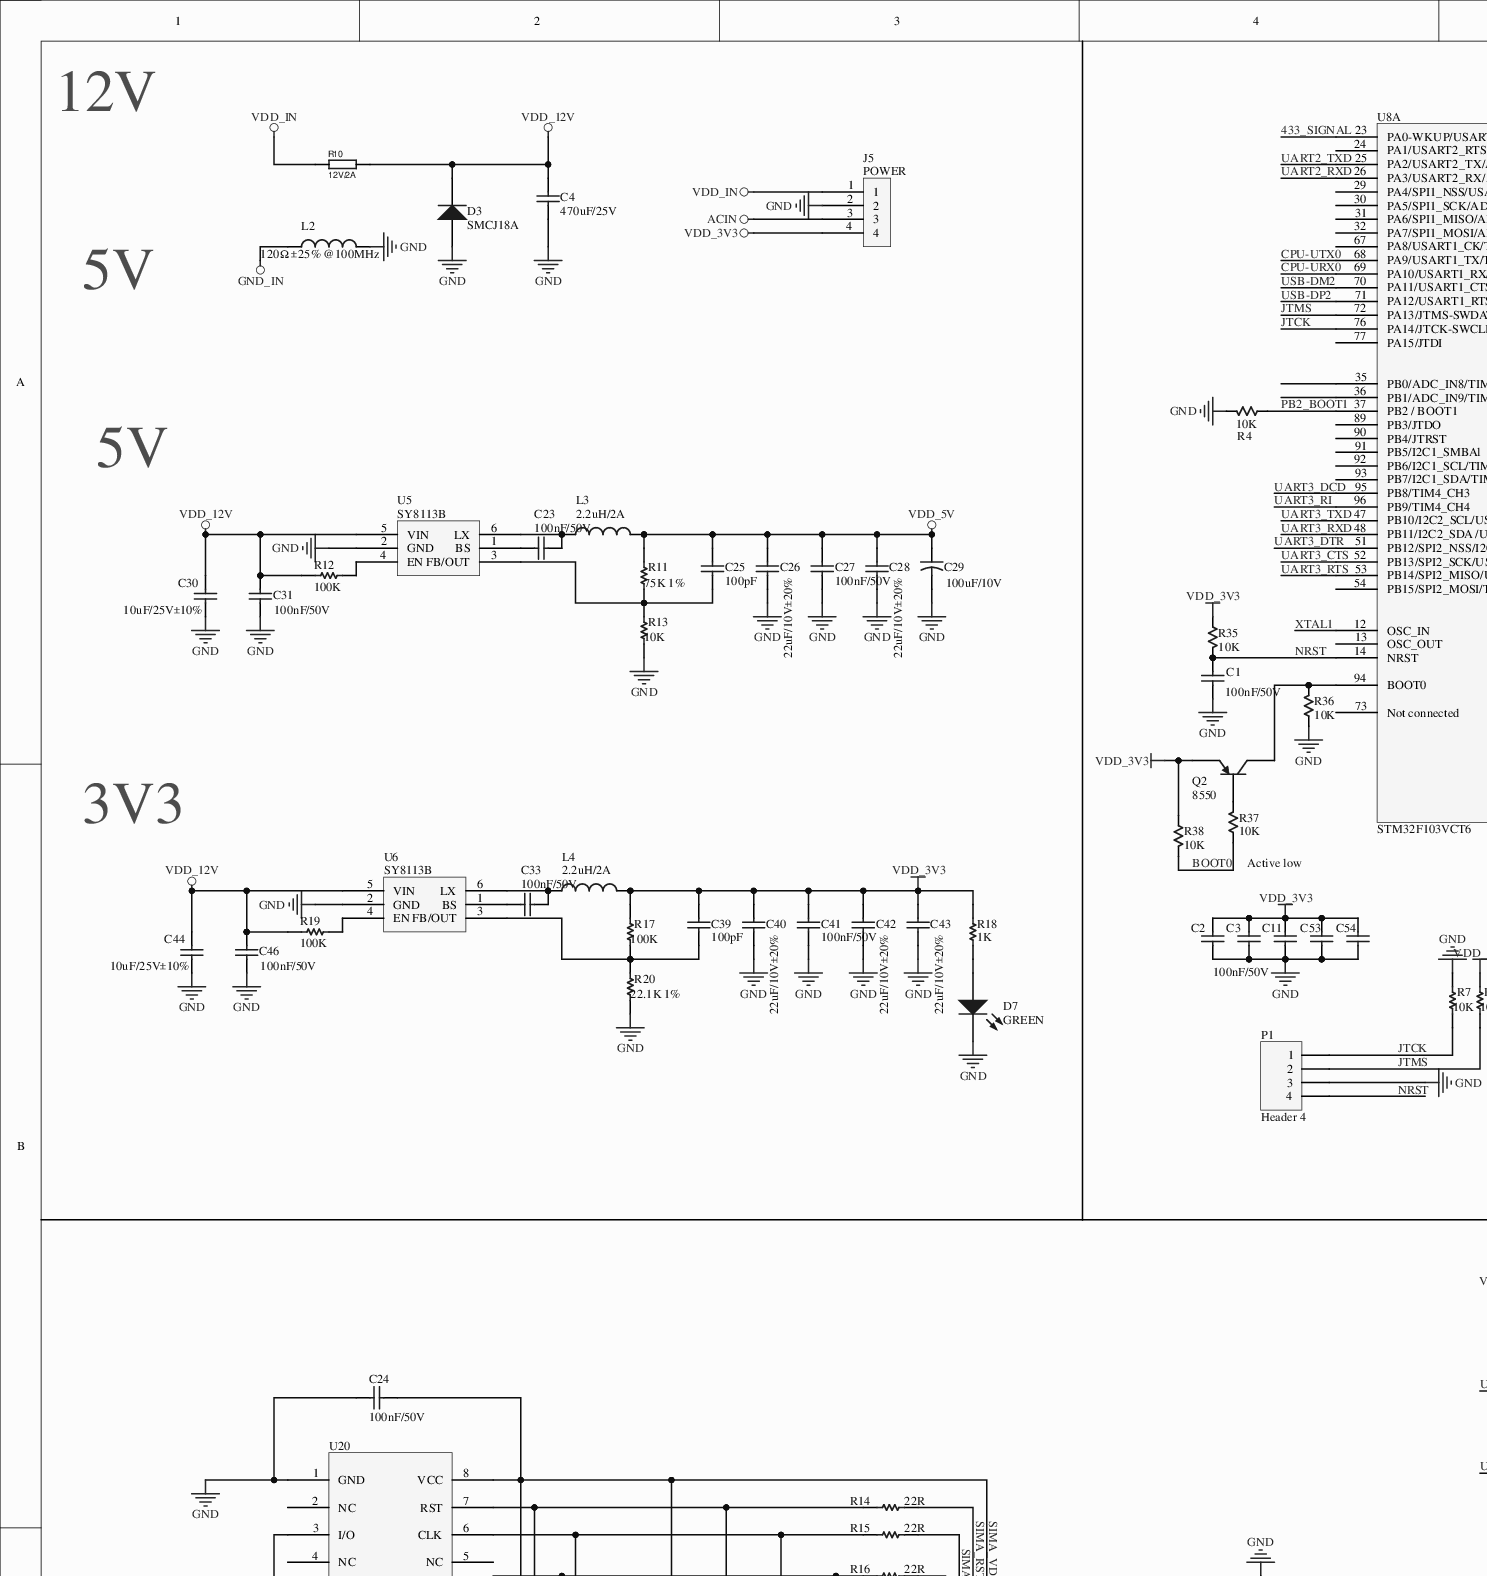
[diagram p0: MISC84456-4.SchDoc, top left]
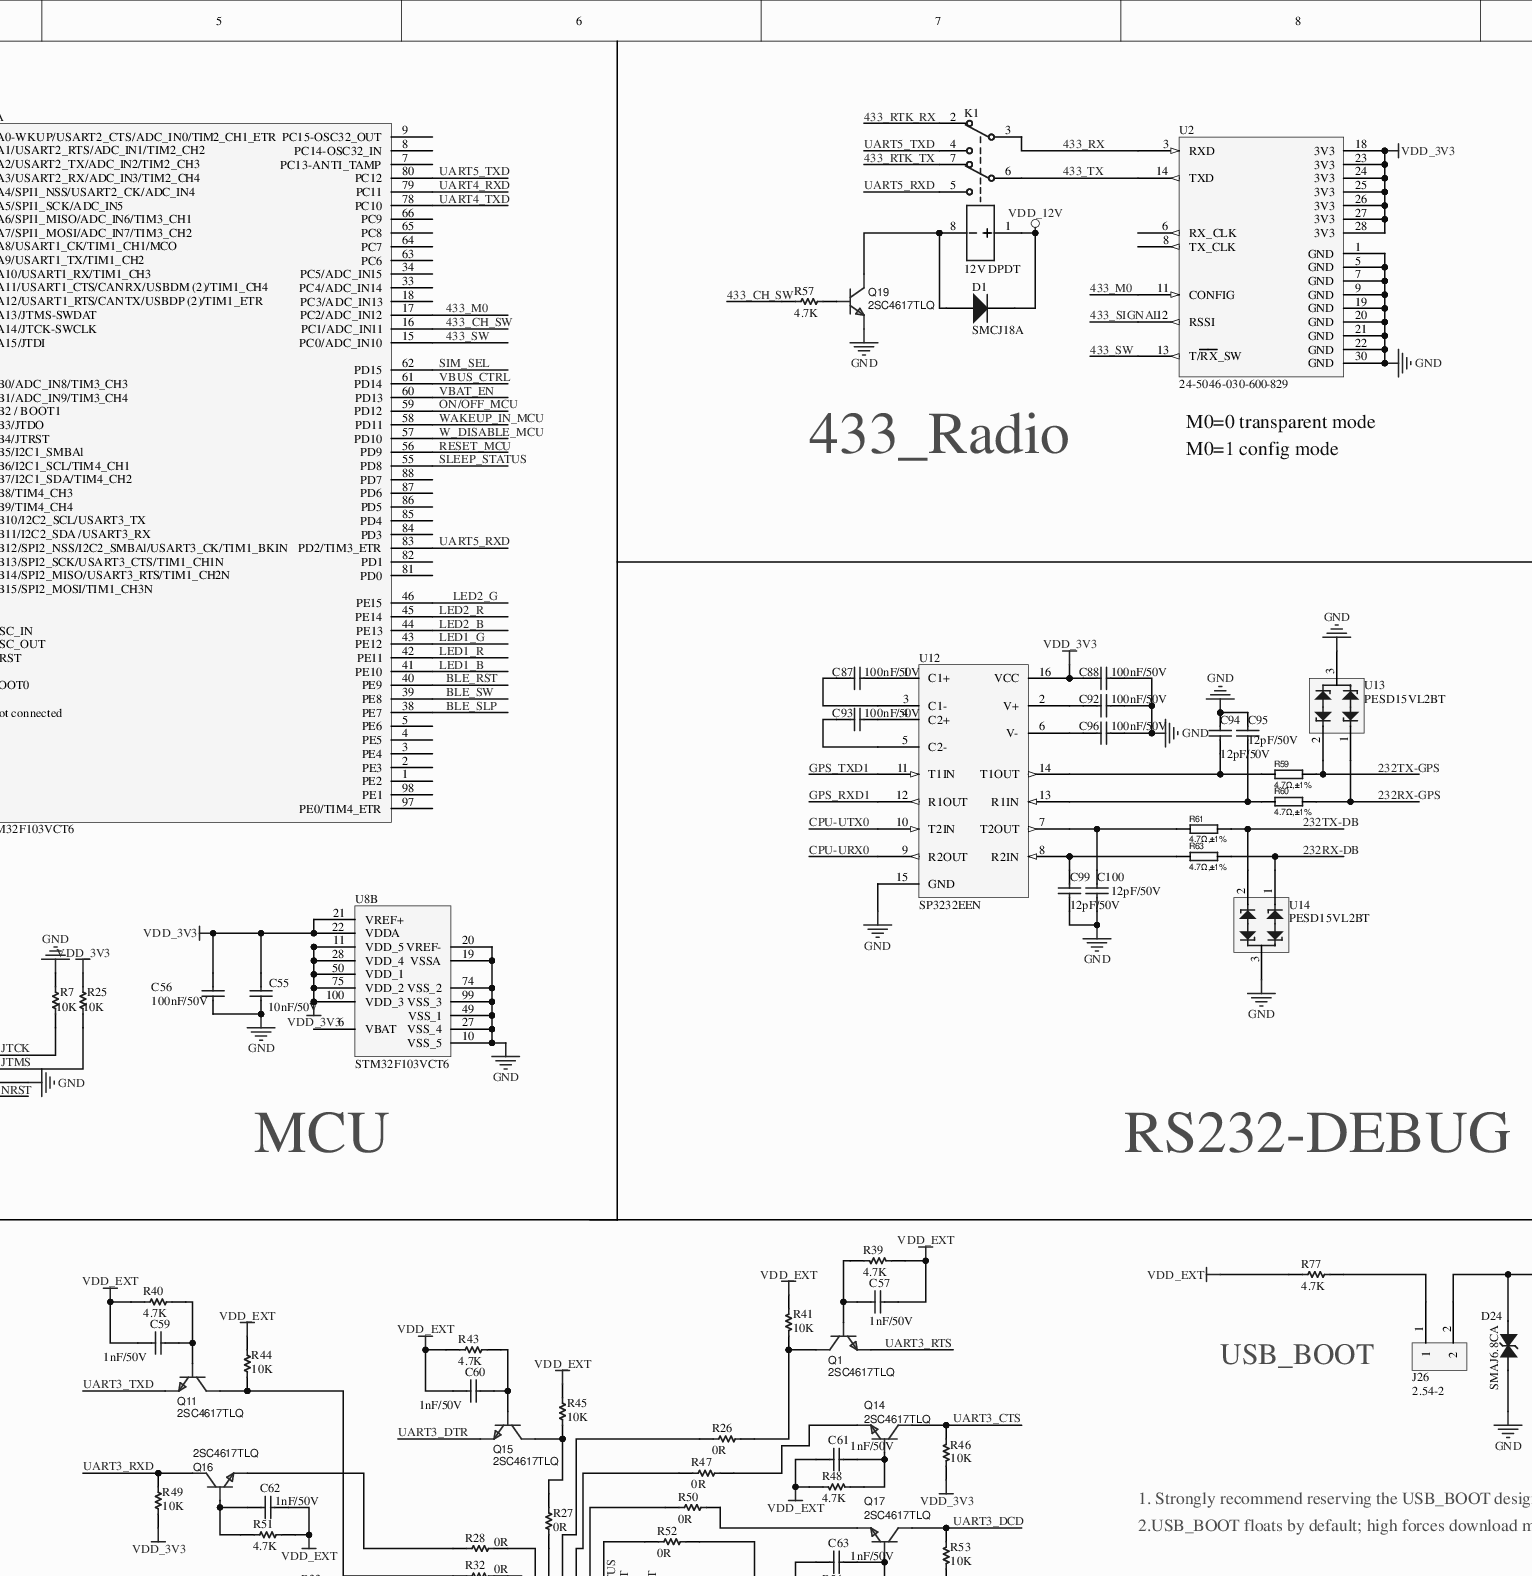
[diagram p1: MISC84456-4.SchDoc, top middle]
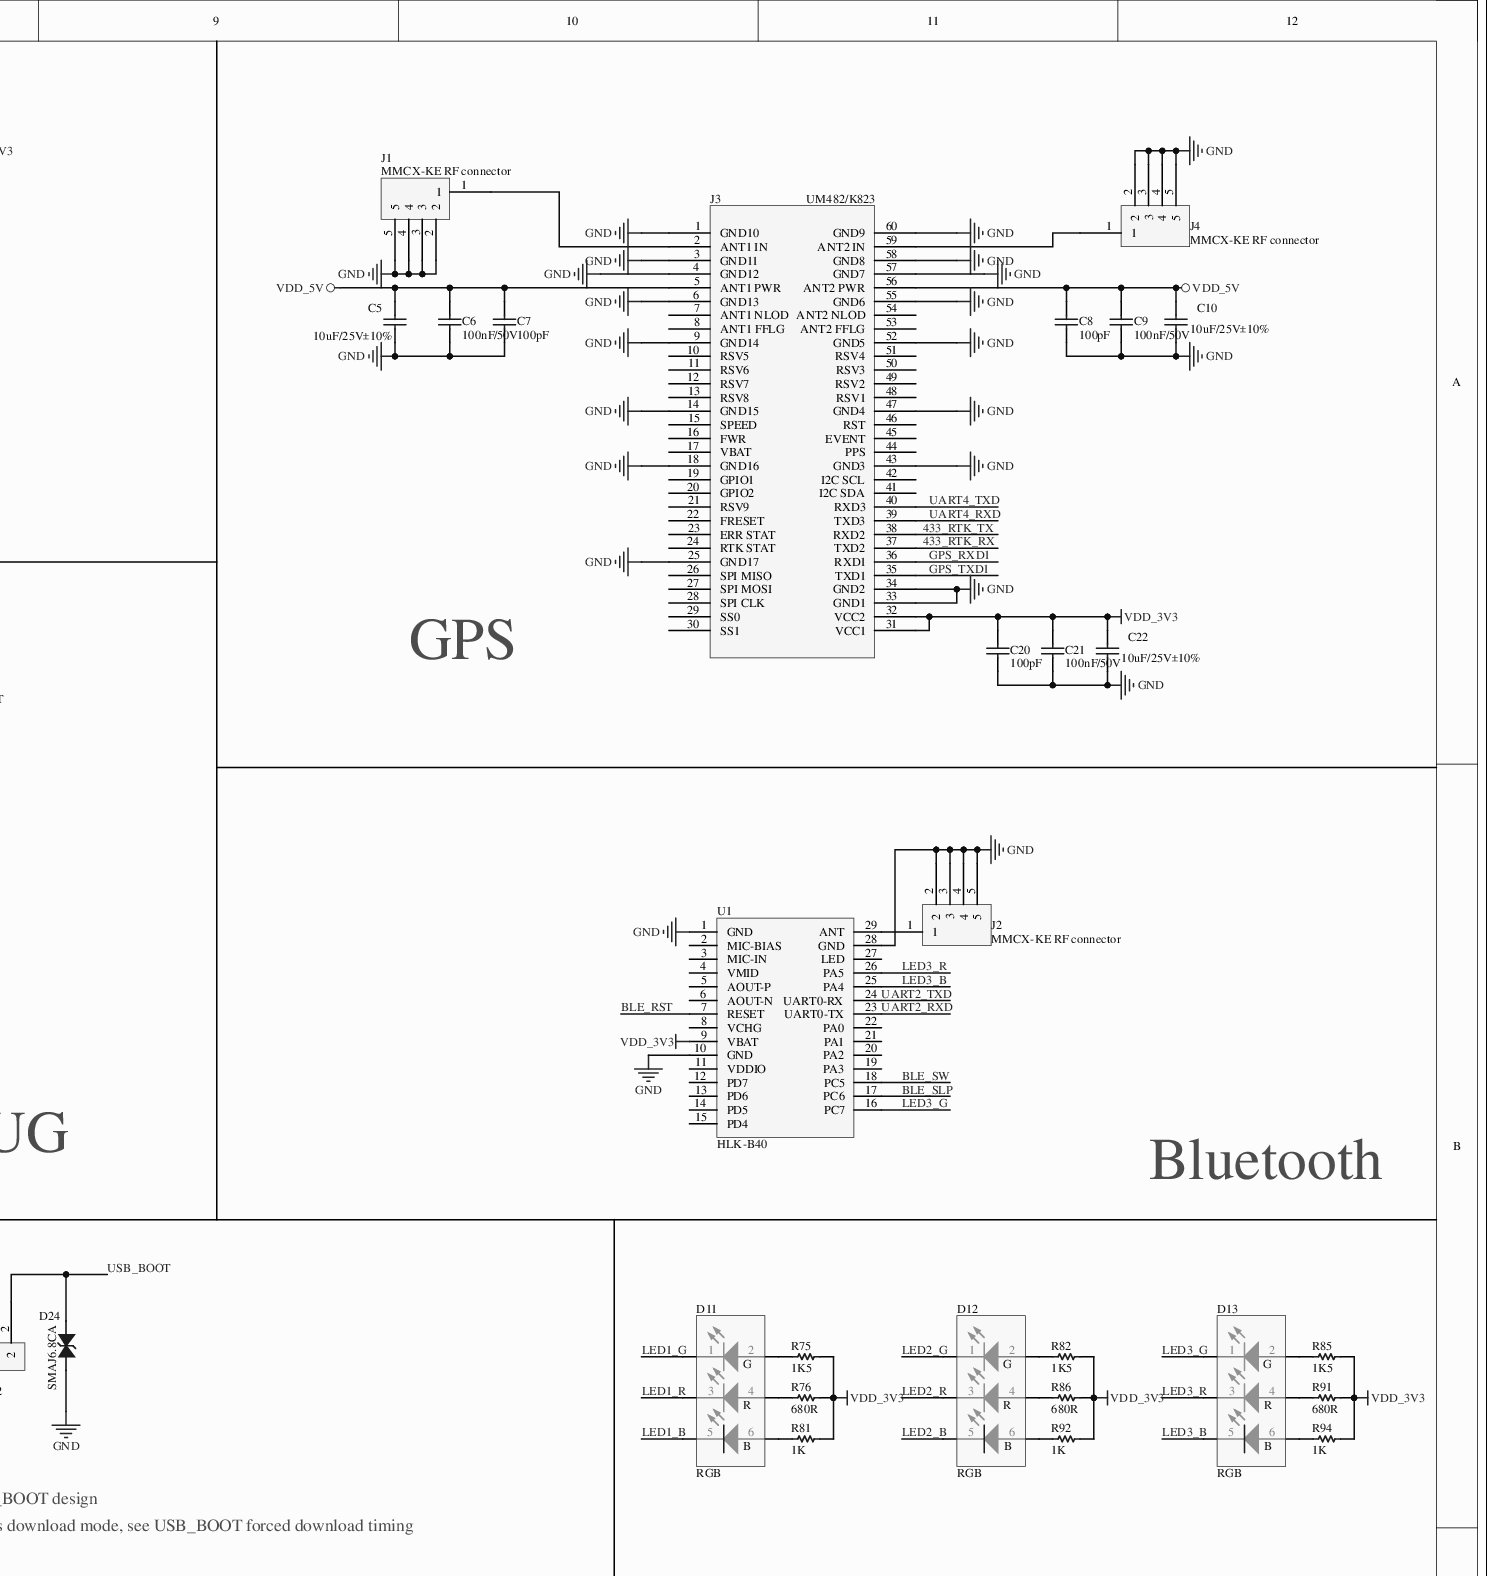
[diagram p2: MISC84456-4.SchDoc, top right]
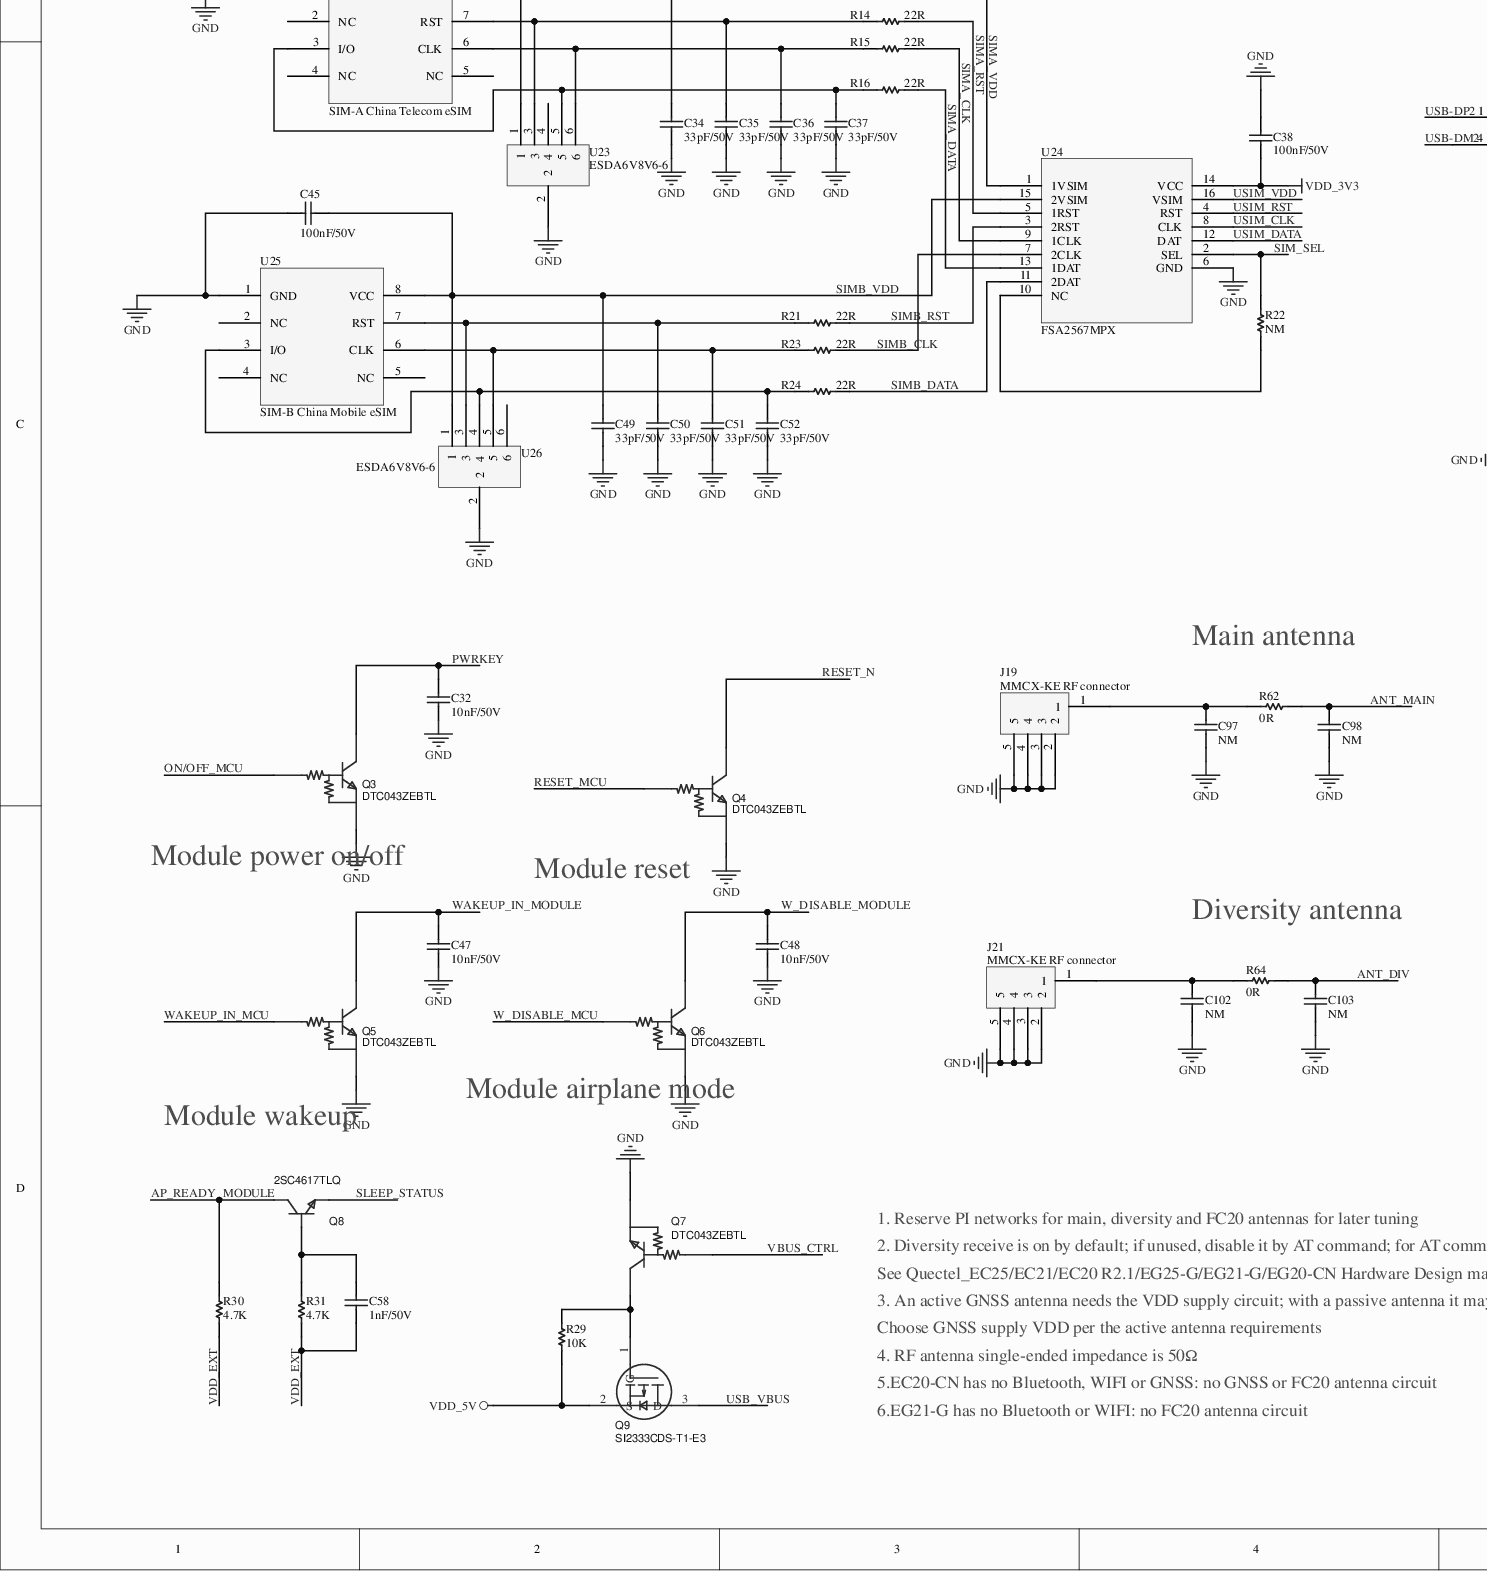
[diagram p3: MISC84456-4.SchDoc, bottom left]
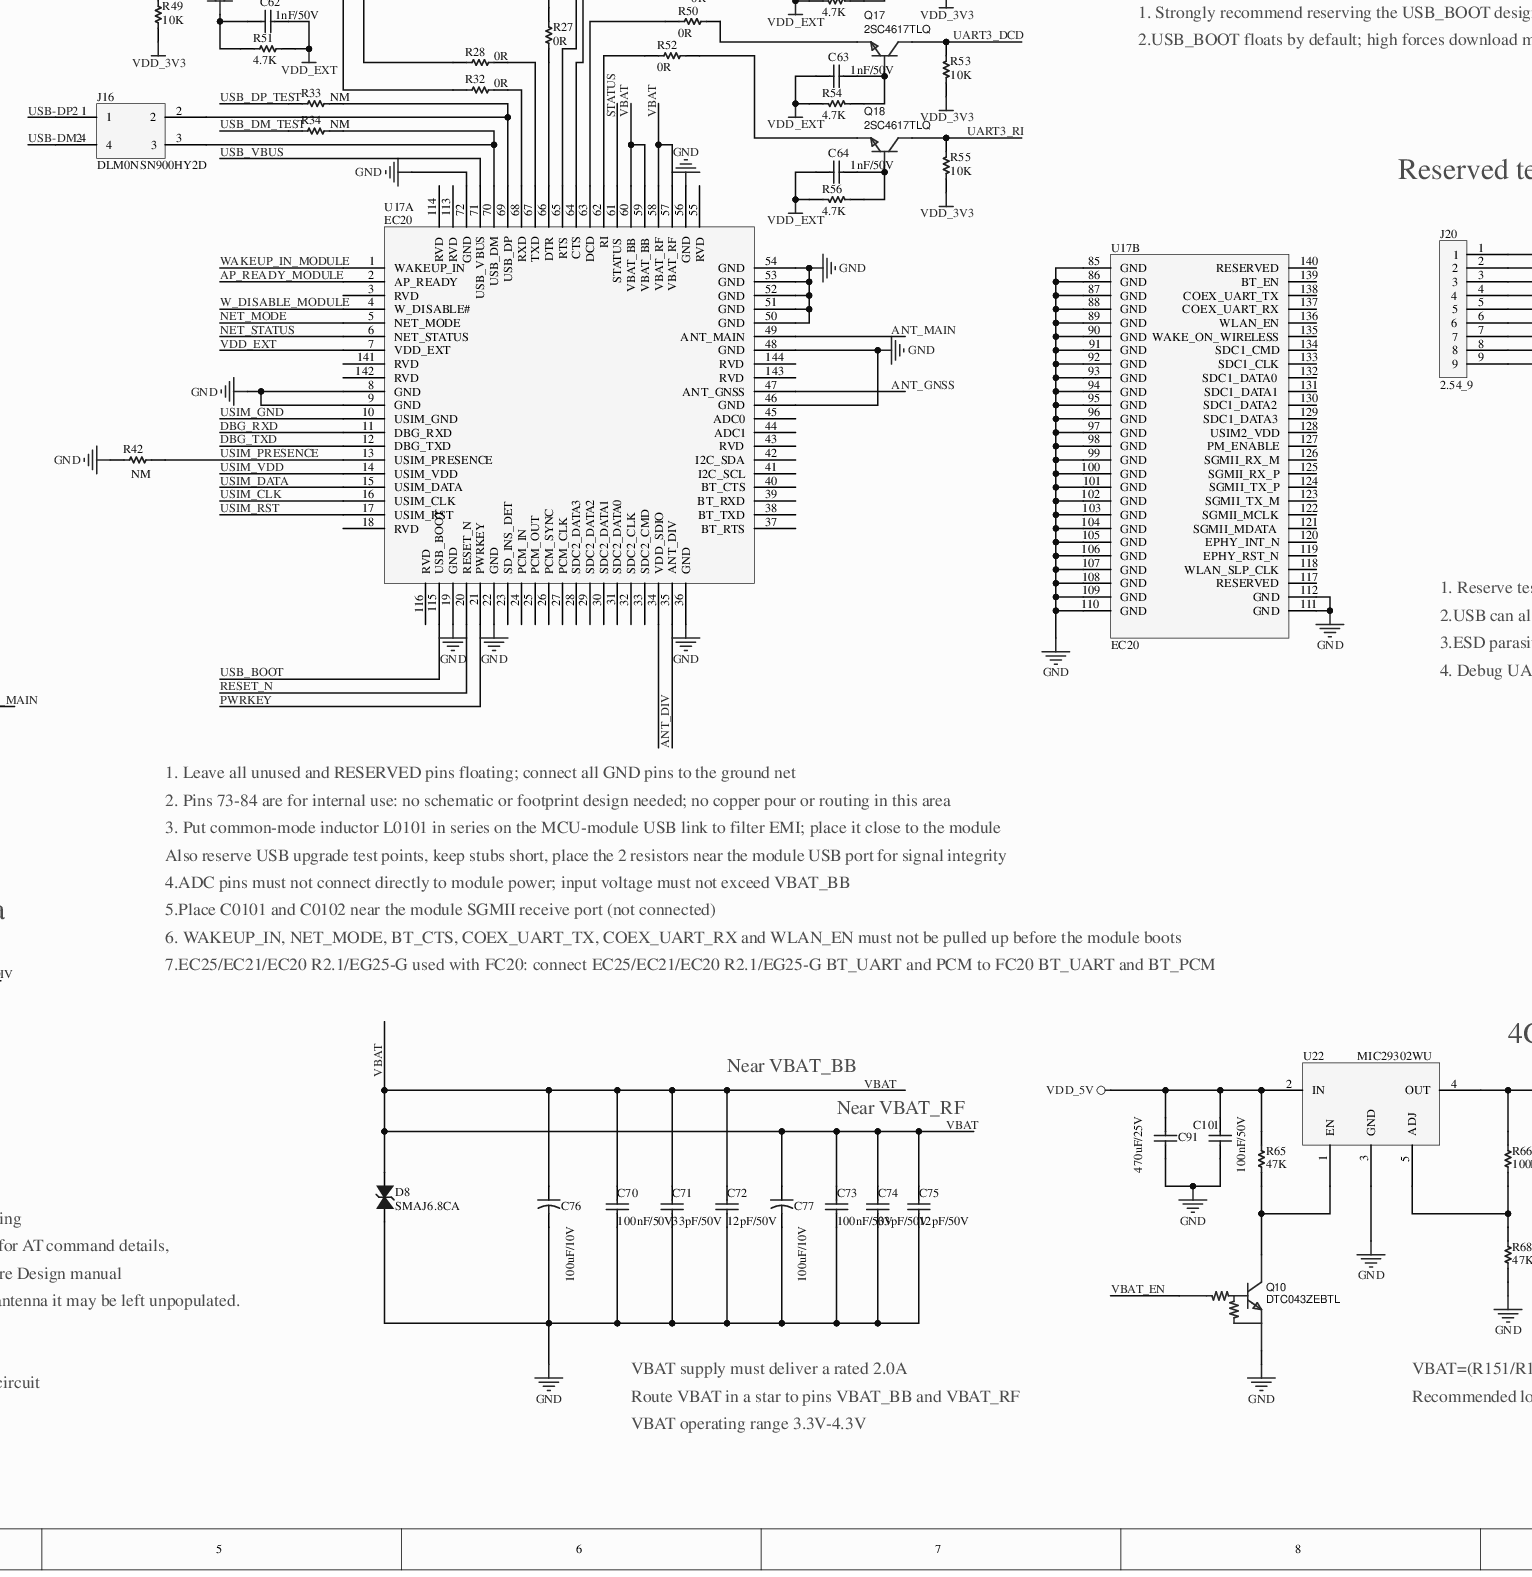
[diagram p4: MISC84456-4.SchDoc, bottom middle]
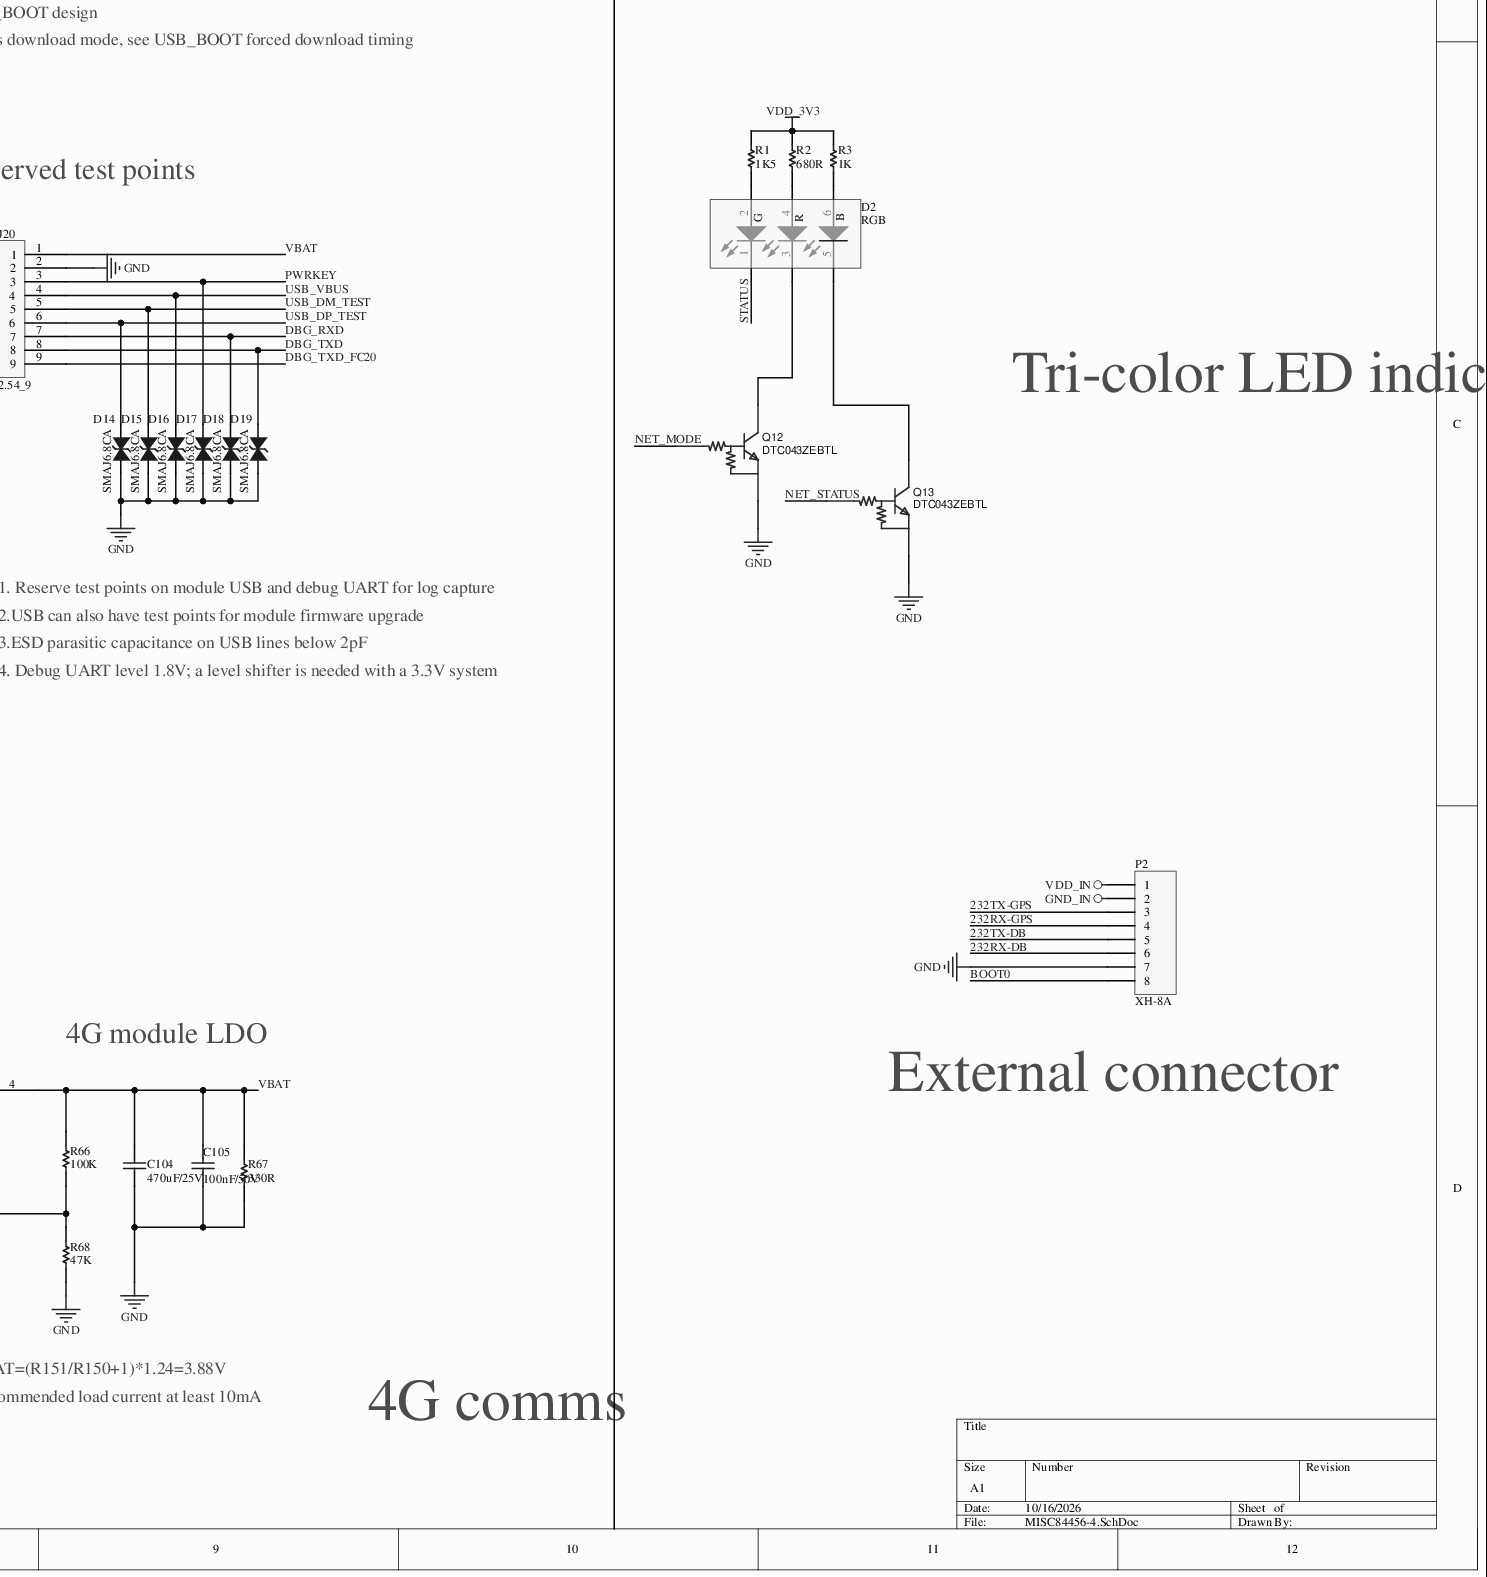
[diagram p5: MISC84456-4.SchDoc, bottom right]
# Altium project MISC84456-3.PrjPcb (part 1 of 2)
1 sheet, 219 parts. Net scope: global (net labels, ports and power ports of the same name join across sheets).
Board file: MISC84456.PcbDoc